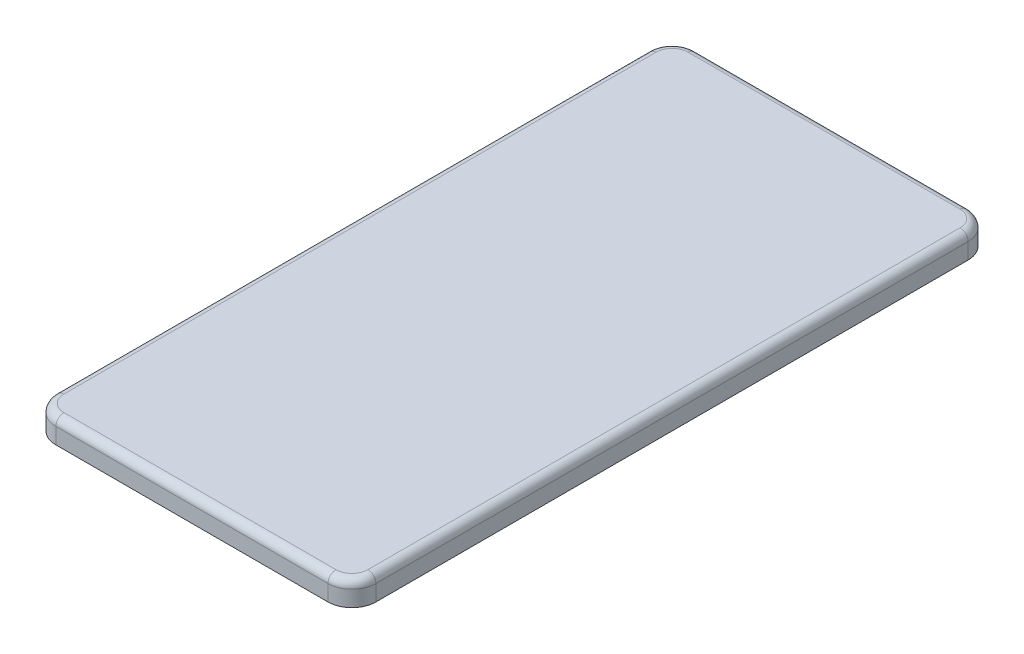
from build123d import *

# Parameters (mm, degrees)
SKETCH_1_W      = 40
SKETCH_1_H      = 80
EXTRUDE_1_DEPTH = 3
FILLET_2_R      = 3
FILLET_3_R      = 1


with BuildPart() as part:
    # 草图1 → 凸台-拉伸1 (new body)
    with BuildSketch(Plane(origin=(0, 0, 0), x_dir=(1, 0, 0), z_dir=(0, 1, 0))):
        Rectangle(SKETCH_1_W, SKETCH_1_H)
    extrude(amount=EXTRUDE_1_DEPTH)

    # 圆角2
    fillet_2_edges = [part.edges().sort_by_distance(p)[0] for p in [
        (20, 1.5, 40),
        (-20, 1.5, 40),
        (-20, 1.5, -40),
        (20, 1.5, -40),
    ]]
    fillet(fillet_2_edges, radius=FILLET_2_R)

    # 圆角3
    fillet_3_edges = [part.edges().sort_by_distance(p)[0] for p in [
        (-20, 3, 0),
        (0, 3, -40),
        (20, 3, 0),
        (0, 3, 40),
        (19.121320344, 3, 39.121320344),
        (-19.121320344, 3, 39.121320344),
        (19.121320344, 3, -39.121320344),
        (-19.121320344, 3, -39.121320344),
    ]]
    fillet(fillet_3_edges, radius=FILLET_3_R)


solid = part.part
